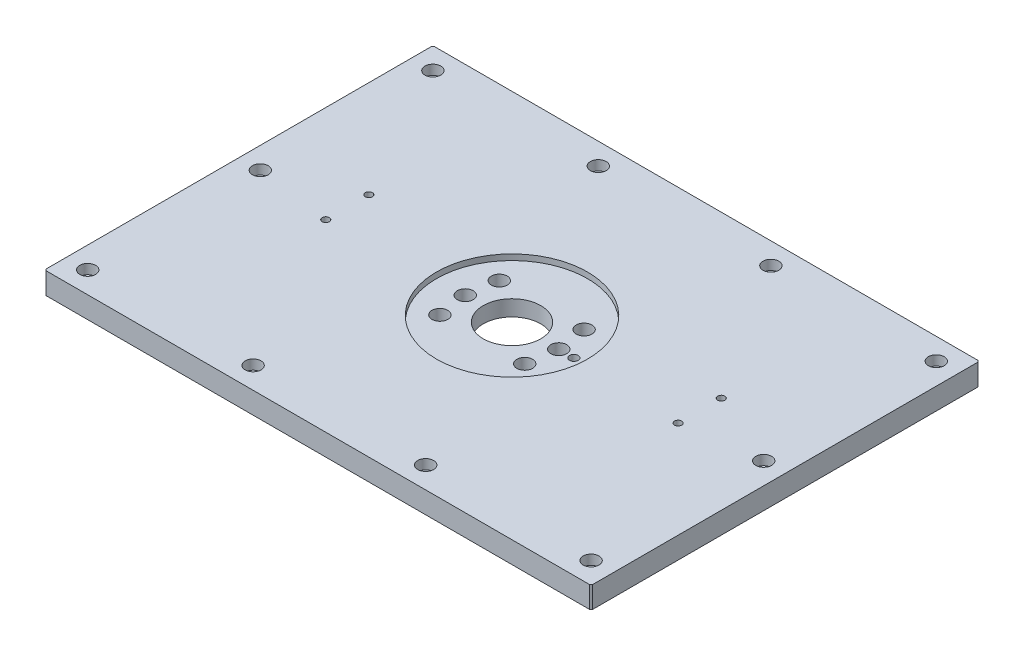
SolidWorks part; units mm, degrees
material "A6061"
ref_plane "前基準面" through (0, 0, 0) normal (0, 0, 1) x (1, 0, 0)
ref_plane "上基準面" through (0, 0, 0) normal (0, 1, 0) x (1, 0, 0)
ref_plane "右基準面" through (0, 0, 0) normal (1, 0, 0) x (0, 0, -1)
sketch "草图1" plane through (0, 0, 0) normal (0, 1, 0) x (1, 0, 0)
  line L1 (-190, -135) -> (190, -135)
  line L2 (-190, -135) -> (-190, 135)
  line L3 (-190, 135) -> (190, 135)
  line L4 (190, -135) -> (190, 135)
  line L5 (-190, -135) -> (190, 135) construction
  line L6 (-190, 135) -> (190, -135) construction
  point P0 (0, 0)
  dimension "D1" = 380
  dimension "D2" = 270
extrude "凸台-拉伸1" add sketch "草图1" along normal mid plane 15
chamfer "倒角1" distance 1 angle 45 4 edges at (190, 0, -135) (190, 0, 135) (-190, 0, -135) (-190, 0, 135)
sketch "草图2" plane through (0, 7.5, 0) normal (0, 1, 0) x (1, 0, 0)
  circle A0 centre (0, 0) radius 20
  dimension "D1" = 40
extrude "切除-拉伸1" cut sketch "草图2" against normal up to surface (15 mm away) up to face at (0, -7.5, 0)
hole_wizard "打孔尺寸(%根据)内六角圆柱头螺钉的类型3" positions "草图4" profile "草图3" counterbore size "M6" standard "GB" end condition through all
sketch "草图4" plane through (0, 7.5, 0) normal (0, 1, 0) x (1, 0, 0)
  line L0 (0, 123.0442) -> (0, 0) construction
  line L1 (0, 0) -> (-143.5202, 0) construction
  line L6 (-190, 134) -> (-190, -134) construction
  point P0 (-175, 120)
  point P4 (-60, 120)
  point P13 (-60, -120)
  point P14 (-175, 0)
  point P15 (-175, -120)
  point P16 (175, -120)
  point P17 (175, 0)
  point P18 (60, -120)
  point P19 (60, 120)
  point P21 (175, 120)
  dimension "D1" = 120
  dimension "D2" = 15
  dimension "D3" = 240
sketch "草图3" plane through (-175, 7.5, -120) normal (1, 0, 0) x (0, 0, 1)
  line L0 (0, 0) -> (0, 15)
  line L1 (0, 15) -> (3.3, 15)
  line L3 (3.3, 15) -> (3.3, 6.8)
  line L4 (3.3, 6.8) -> (5.5, 6.8)
  line L5 (5.5, 6.8) -> (5.5, 0)
  line L7 (5.5, 0) -> (0, 0)
  line L11 (0, -6.35) -> (0, 107.95) construction
  dimension "通孔孔直径" = 6.6
  dimension "通孔孔深度" = 15
  dimension "柱形沉头孔直径" = 11
  dimension "柱形沉头孔深度" = 6.8
sketch "草图9" plane through (0, 7.5, 0) normal (0, 1, 0) x (1, 0, 0)
  line L0 (0, 0) -> (-29.4895, 20.6488) construction
  line L3 (0, 0) -> (23.4885, 0) construction
  line L4 (0, 0) -> (-32.5, 0) construction
  line L5 (0, 0) -> (-29.4895, -20.6488) construction
  line L6 (0, 0) -> (0, 17.9329) construction
  line L7 (-32.5, 0) -> (-43, 0) construction
  circle A1 centre (0, 0) radius 36 construction
  circle A4 centre (-29.4895, 20.6488) radius 5.5
  circle A5 centre (-29.4895, -20.6488) radius 5.5
  circle A6 centre (-32.5, 0) radius 5.5
  circle A7 centre (29.4895, -20.6488) radius 5.5
  circle A8 centre (32.5, 0) radius 5.5
  circle A9 centre (29.4895, 20.6488) radius 5.5
  dimension "D1" = 72
  dimension "D4" = 11
  dimension "D2" = 35
  dimension "D3" = 32.5
extrude "切除-拉伸2" cut sketch "草图9" against normal through all
sketch "草图10" plane through (0, 7.5, 0) normal (0, 1, 0) x (1, 0, 0)
  circle A0 centre (0, 0) radius 52.5
  dimension "D1" = 105
sketch "草图11" plane through (0, 7.5, 0) normal (0, 1, 0) x (1, 0, 0)
  circle A0 centre (0, 0) radius 52.5
  dimension "D1" = 105
extrude "切除-拉伸3" cut sketch "草图11" against normal blind 4
hole_wizard "M6 螺纹孔1" positions "草图12" profile "草图13" tap size "M6" standard "GB" end condition through all
sketch "草图12" plane through (0, 7.5, 0) normal (0, 1, 0) x (1, 0, 0)
  line L0 (0, 0) -> (0, 83.8877) construction
  point P0 (122.5, -7)
  point P3 (122.5, 23)
  point P12 (-122.5, 23)
  point P13 (-122.5, -7)
sketch "草图13" plane through (122.5, 7.5, 7) normal (1, 0, 0) x (0, 0, 1)
  line L0 (0, 0) -> (0, 15)
  line L1 (0, 15) -> (2.5, 15)
  line L2 (2.5, 15) -> (2.5, 0)
  line L5 (2.5, 0) -> (0, 0)
  line L11 (0, -6.35) -> (0, 107.95) construction
  dimension "通孔螺纹孔钻头直径" = 5
  dimension "通孔螺纹孔钻头深度" = 15
cosmetic thread "孔螺蚊线1" parameters "D2"=6
cosmetic thread "孔螺蚊线2" parameters "D2"=6
cosmetic thread "孔螺蚊线3" parameters "D2"=6
cosmetic thread "孔螺蚊线4" parameters "D2"=6
sketch "草图15" plane through (0, 3.5, 0) normal (0, 1, 0) x (1, 0, 0)
  line L0 (0, 0) -> (43, 0) construction
  circle A0 centre (43, 0) radius 3
  dimension "D2" = 6
  dimension "D1" = 43
extrude "切除-拉伸4" cut sketch "草图15" against normal blind 9
equation "\"D3@草图6\"=\"D2@草图6\""
